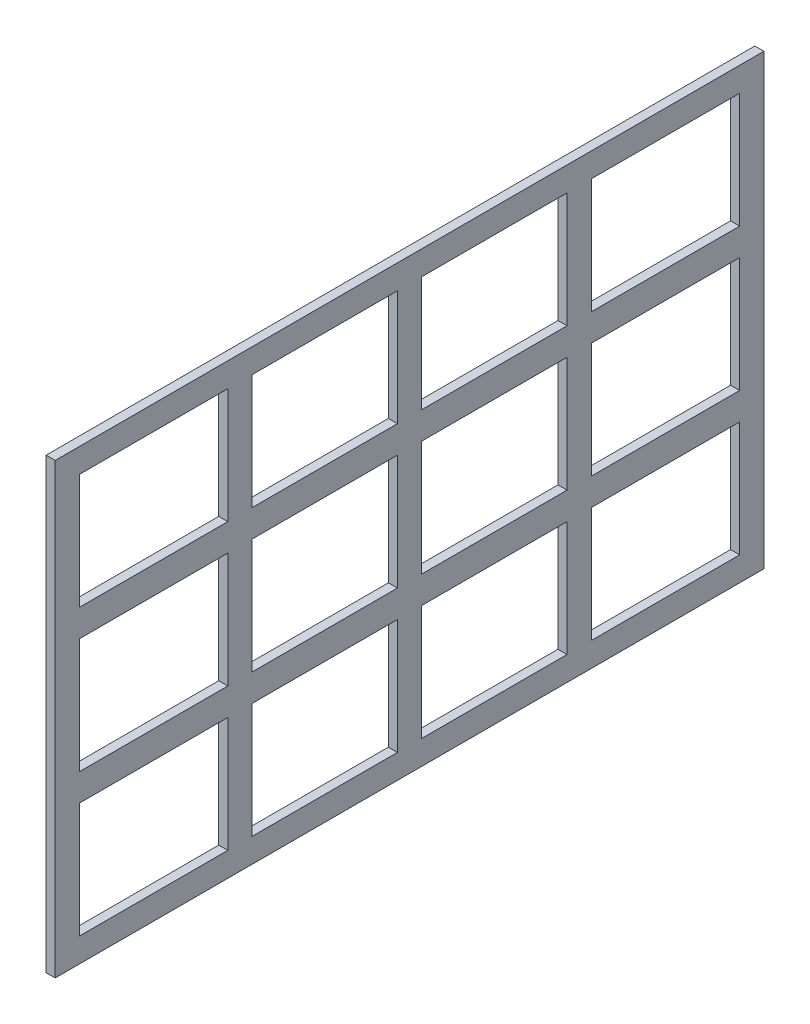
SolidWorks part; units mm, degrees
material "Q235-A"
ref_plane "Front Plane" through (0, 0, 0) normal (0, 0, 1) x (1, 0, 0)
ref_plane "Top Plane" through (0, 0, 0) normal (0, 1, 0) x (1, 0, 0)
ref_plane "Right Plane" through (0, 0, 0) normal (1, 0, 0) x (0, 0, -1)
sketch "Sketch1" plane through (0, 0, 0) normal (1, 0, 0) x (0, 0, -1)
  line L1 (585, -370) -> (-585, -370)
  line L2 (585, -370) -> (585, 370)
  line L3 (585, 370) -> (-585, 370)
  line L4 (-585, -370) -> (-585, 370)
  line L5 (585, -370) -> (-585, 370) construction
  line L6 (585, 370) -> (-585, -370) construction
  point P0 (0, 0)
  dimension "D1" = 1170
  dimension "D2" = 740
extrude "Boss-Extrude1" add sketch "Sketch1" along normal mid plane 15
sketch "Sketch2" plane through (7.5, 0, 0) normal (1, 0, 0) x (0, 0, -1)
  line L0 (0, -510.8451) -> (0, 510.8451) construction
  line L1 (665.7465, 0) -> (-665.7465, 0) construction
  line L2 (-585, 370) -> (-585, -370) construction
  line L3 (-545, 330) -> (-300, 330)
  line L4 (-545, 330) -> (-545, 140)
  line L5 (-545, 140) -> (-300, 140)
  line L6 (-300, 330) -> (-300, 140)
  line L7 (-545, 330) -> (-300, 140) construction
  line L8 (-545, 140) -> (-300, 330) construction
  line L9 (-545, 95) -> (-300, 95)
  line L10 (-545, 95) -> (-545, -95)
  line L11 (-545, -95) -> (-300, -95)
  line L12 (-300, 95) -> (-300, -95)
  line L13 (-260, 95) -> (-20, 95)
  line L14 (-260, 95) -> (-260, -95)
  line L15 (-260, 330) -> (-20, 330)
  line L16 (-260, 330) -> (-260, 140)
  line L17 (-260, 140) -> (-20, 140)
  line L18 (-20, 330) -> (-20, 140)
  line L19 (-260, 330) -> (-20, 140) construction
  line L20 (-260, 140) -> (-20, 330) construction
  line L21 (585, 370) -> (-585, 370) construction
  line L22 (-260, -95) -> (-20, -95)
  line L23 (-20, 95) -> (-20, -95)
  line L24 (-545, 95) -> (-300, -95) construction
  line L25 (-545, -95) -> (-300, 95) construction
  line L26 (-260, 95) -> (-20, -95) construction
  line L27 (-260, -95) -> (-20, 95) construction
  line L28 (-545, -140) -> (-300, -140)
  line L29 (-545, -140) -> (-545, -330)
  line L30 (-545, -330) -> (-300, -330)
  line L31 (-300, -140) -> (-300, -330)
  line L32 (-260, -140) -> (-20, -140)
  line L33 (-260, -140) -> (-260, -330)
  line L34 (-260, -330) -> (-20, -330)
  line L35 (-20, -140) -> (-20, -330)
  line L36 (-545, -140) -> (-300, -330) construction
  line L37 (-545, -330) -> (-300, -140) construction
  line L38 (-260, -140) -> (-20, -330) construction
  line L39 (-260, -330) -> (-20, -140) construction
  point P0 (-422.5, 235)
  point P4 (0, 0)
  point P8 (0, 0)
  point P14 (-422.5, 0)
  point P18 (-140, 235)
  point P28 (-140, 0)
  point P33 (-422.5, -235)
  point P38 (-140, -235)
  dimension "D1" = 20
  dimension "D2" = 40
  dimension "D3" = 3
  dimension "D4" = 240
  dimension "D5" = 40
  dimension "D6" = 40
  dimension "D7" = 190
extrude "Cut-Extrude1" cut sketch "Sketch2" against normal blind 108
mirror "Mirror1" about plane through (0, 0, 0) normal (0, 0, 1) of "Cut-Extrude1"
